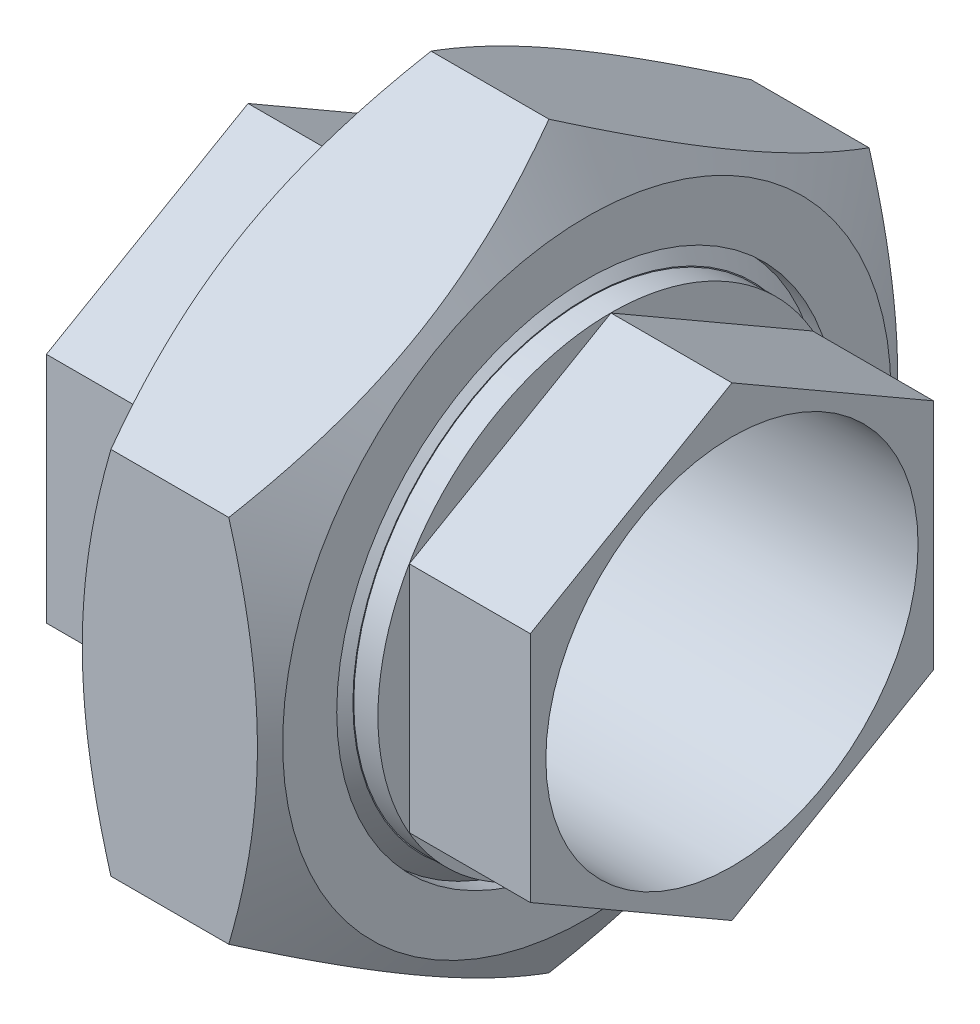
from build123d import *

# Parameters (mm, degrees)
CHAMFER_1_SIZE           = 2.606
CUT_EXTRUDE_START        = -19.5
SKETCH_4_R               = 40.3075
CUT_EXTRUDE_1_DEPTH      = 19.5
SKETCH_8_R               = 65.5435
CUT_EXTRUDE_3_DEPTH      = 101.408687124
SKETCH_10_OUTSIDE_W      = 175.022
SKETCH_10_OUTSIDE_H      = 190.988
SKETCH_10_OUTSIDE_R      = 49.0220175
CUT_EXTRUDE_4_DEPTH      = 10
CUT_EXTRUDE_4_DRAFT      = -60
MIRROR_7_COPY_1_SKETCH_W = 175.022
MIRROR_7_COPY_1_SKETCH_H = 190.988
MIRROR_7_COPY_1_SKETCH_R = 49.0220175
MIRROR_7_COPY_1_DEPTH    = 10
MIRROR_7_COPY_1_DRAFT    = -60
SKETCH_11_R              = 30
CUT_EXTRUDE_5_DEPTH      = 111.892521812
SKETCH_12_R              = 30
EXTRUDE_1_DEPTH          = 19.5
SKETCH_13_R              = 37.558920999
SKETCH_13_R_2            = 35.05
EXTRUDE_2_DEPTH          = 35.1


with BuildPart() as part:
    # 草图1 → 旋转1 (revolve)
    with BuildSketch(Plane.XY, mode=Mode.PRIVATE) as revolve_1_sk:
        Polygon((39, 35.05), (15.6, 35.05), (15.6, 40.3075), (0, 40.3075), (0, 46.266), (-15.6, 46.266), (-15.6, 35.05), (-39, 35.05), (-39, 26.877146006), (-15.6, 26.06), (15.6, 26.06), (39, 26.877146006), align=None)
    revolve(revolve_1_sk.sketch.rotate(Axis((0, 0, 0), (1, 0, 0)), 90), axis=Axis((0, 0, 0), (1, 0, 0)))

    # 倒角1
    chamfer_1_edges = [part.edges().sort_by_distance(p)[0] for p in [
        (-15.6, 0, -46.266),
        (15.6, 0, -40.3075),
    ]]
    chamfer(chamfer_1_edges, length=CHAMFER_1_SIZE)

    # 草图3 → 旋转2 (revolve)
    with BuildSketch(Plane.XY, mode=Mode.PRIVATE) as revolve_2_sk:
        Polygon((-15.6, 46.266), (-15.6, 59.585), (15.6, 59.585), (15.6, 40.3075), (0, 40.3075), (0, 46.266), align=None)
    revolve(revolve_2_sk.sketch.rotate(Axis((0, 0, 0), (1, 0, 0)), 90), axis=Axis((0, 0, 0), (1, 0, 0)))

    # 草图4 → 切除-拉伸1 (cut)
    with BuildSketch(Plane(origin=(39, 0, 0), x_dir=(0, 0, -1), z_dir=(1, 0, 0)).offset(CUT_EXTRUDE_START)):
        with Locations(Location((0, 0, 0), (0, 0, 180))):
            Circle(SKETCH_4_R)
        Polygon((0, 35.05), (-30.354190403, 17.525), (-30.354190403, -17.525), (0, -35.05), (30.354190403, -17.525), (30.354190403, 17.525), align=None, mode=Mode.SUBTRACT)
    cut_extrude_1 = extrude(amount=CUT_EXTRUDE_1_DEPTH, mode=Mode.SUBTRACT)

    # 草图6 → 旋转3 (revolve)
    with BuildSketch(Plane.XY, mode=Mode.PRIVATE) as revolve_3_sk:
        with BuildLine():
            Line((25.472011753, 26.404738247), (15.6, 26.404738247))
            Line((15.6, 26.404738247), (15.6, 36.27675))
            ThreePointArc((15.6, 36.27675), (18.491445299, 29.296183545), (25.472011753, 26.404738247))
        make_face()
    revolve_3 = revolve(revolve_3_sk.sketch.rotate(Axis((0, 0, 0), (1, 0, 0)), 120), axis=Axis((0, 0, 0), (1, 0, 0)))

    # 草图8 → 切除-拉伸3 (cut, through all)
    with BuildSketch(Plane(origin=(15.6, 0, 0), x_dir=(0, 0, -1), z_dir=(1, 0, 0))):
        Circle(SKETCH_8_R)
        Polygon((0, 59.585), (-51.602123684, 29.7925), (-51.602123684, -29.7925), (0, -59.585), (51.602123684, -29.7925), (51.602123684, 29.7925), align=None, mode=Mode.SUBTRACT)
    extrude(amount=-CUT_EXTRUDE_3_DEPTH, mode=Mode.SUBTRACT)


with BuildPart() as cut_extrude_4_tool:
    # 草图10 outside → 切除-拉伸4 (with draft: the straight prism first)
    with BuildSketch(Plane(origin=(15.6, 0, 0), x_dir=(0, 0, -1), z_dir=(1, 0, 0))):
        Rectangle(SKETCH_10_OUTSIDE_W, SKETCH_10_OUTSIDE_H)
        Circle(SKETCH_10_OUTSIDE_R, mode=Mode.SUBTRACT)
    extrude(amount=-CUT_EXTRUDE_4_DEPTH)
    # 切除-拉伸4: the draft: its side faces are tilted about the plane it starts from
    cut_extrude_4_sides = [cut_extrude_4_tool.faces().sort_by_distance(p)[0] for p in [
        (10.6, -95.494, 0),
        (10.6, 0, -87.511),
        (10.6, 95.494, 0),
        (10.6, 0, 87.511),
        (10.6, 0, 49.0220175),
    ]]
    draft(cut_extrude_4_sides, Plane(origin=(15.6, 0, 0), x_dir=(0, 0, -1), z_dir=(1, 0, 0)), CUT_EXTRUDE_4_DRAFT)


with BuildPart() as part_1:
    add(part.part)

    # 切除-拉伸4: cut by cut_extrude_4_tool
    add(cut_extrude_4_tool.part, mode=Mode.SUBTRACT)

    # 镜向7: 切除-拉伸1, 旋转3 across plane
    add(cut_extrude_1.mirror(Plane(origin=(0, 0, 0), x_dir=(0, 0, 1), z_dir=(1, 0, 0))), mode=Mode.SUBTRACT)
    add(revolve_3.mirror(Plane(origin=(0, 0, 0), x_dir=(0, 0, 1), z_dir=(1, 0, 0))))


with BuildPart() as mirror_7_copy_1_tool:
    # 镜向7 copy 1 sketch → 镜向7 copy 1 (with draft: the straight prism first)
    with BuildSketch(Plane(origin=(-15.6, 0, 0), x_dir=(0, 0, -1), z_dir=(-1, 0, 0))):
        Rectangle(MIRROR_7_COPY_1_SKETCH_W, MIRROR_7_COPY_1_SKETCH_H)
        Circle(MIRROR_7_COPY_1_SKETCH_R, mode=Mode.SUBTRACT)
    extrude(amount=-MIRROR_7_COPY_1_DEPTH)
    # 镜向7 copy 1: the draft: its side faces are tilted about the plane it starts from
    mirror_7_copy_1_sides = [mirror_7_copy_1_tool.faces().sort_by_distance(p)[0] for p in [
        (-10.6, -95.494, 0),
        (-10.6, 0, -87.511),
        (-10.6, 95.494, 0),
        (-10.6, 0, 87.511),
        (-10.6, 0, 49.0220175),
    ]]
    draft(mirror_7_copy_1_sides, Plane(origin=(-15.6, 0, 0), x_dir=(0, 0, -1), z_dir=(-1, 0, 0)), MIRROR_7_COPY_1_DRAFT)


with BuildPart() as part_2:
    add(part_1.part)

    # 镜向7 copy 1: cut by mirror_7_copy_1_tool
    add(mirror_7_copy_1_tool.part, mode=Mode.SUBTRACT)

    # 草图11 → 切除-拉伸5 (cut, through all)
    with BuildSketch(Plane.ZY.offset(39)):
        Circle(SKETCH_11_R)
    extrude(amount=-CUT_EXTRUDE_5_DEPTH, mode=Mode.SUBTRACT)

    # 草图12 → 凸台-拉伸1 (add)
    with BuildSketch(Plane.ZY.offset(39)):
        Polygon((0, 37.527767497), (-32.5, 18.763883749), (-32.5, -18.763883749), (0, -37.527767497), (32.5, -18.763883749), (32.5, 18.763883749), align=None)
        Circle(SKETCH_12_R, mode=Mode.SUBTRACT)
    extrude_1 = extrude(amount=-EXTRUDE_1_DEPTH)

    # 草图13 → 凸台-拉伸2 (add)
    with BuildSketch(Plane.ZY.offset(19.5)):
        Circle(SKETCH_13_R)
        with Locations(Location((0, 0, 0), (0, 0, 330))):
            Circle(SKETCH_13_R_2, mode=Mode.SUBTRACT)
    extrude_2 = extrude(amount=-EXTRUDE_2_DEPTH)

    # 镜向8: 凸台-拉伸1, 凸台-拉伸2 across plane
    add(extrude_1.mirror(Plane(origin=(0, 0, 0), x_dir=(0, 0, 1), z_dir=(1, 0, 0))))
    add(extrude_2.mirror(Plane(origin=(0, 0, 0), x_dir=(0, 0, 1), z_dir=(1, 0, 0))))


solid = part_2.part
